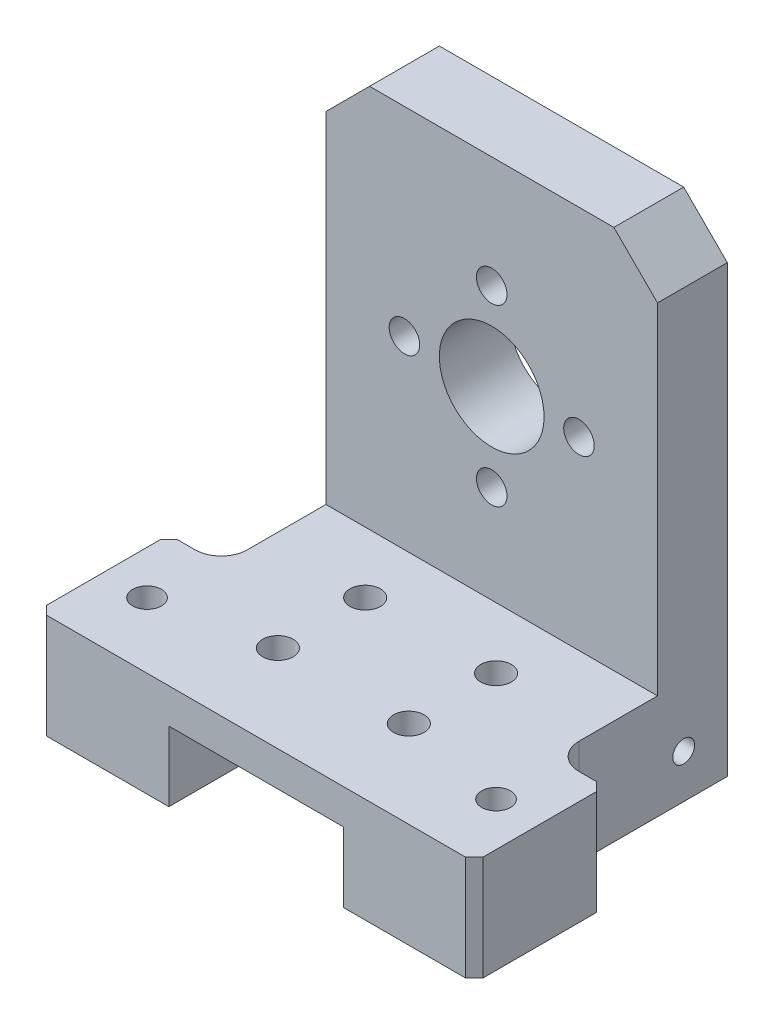
from build123d import *

# Parameters (mm, degrees)
SKETCH1_W             = 50
SKETCH1_H             = 56
SKETCH1_R             = 6
BOSS_EXTRUDE1_DEPTH   = 8
SKETCH2_W             = 50
SKETCH2_H             = 35
BOSS_EXTRUDE2_DEPTH   = 12
SKETCH3_W             = 20
SKETCH3_H             = 35
CUT_EXTRUDE1_DEPTH    = 8
SKETCH4_W             = 6
SKETCH4_H             = 44
CUT_EXTRUDE2_DEPTH    = 60
CHAMFER2_SIZE         = 5
SKETCH5_W             = 6
SKETCH5_H             = 20
CUT_EXTRUDE3_DEPTH    = 60
M4_TAPPED_HOLE1_D     = 3.3
FILLET1_R             = 3
SKETCH9_R             = 1.75
CUT_EXTRUDE4_DEPTH    = 10
SKETCH10_R            = 1.75
CUT_EXTRUDE5_DEPTH    = 10
M3_TAPPED_HOLE1_D     = 2.5
M3_TAPPED_HOLE1_DEPTH = 7.5
M3_TAPPED_HOLE1_TIP   = 0.751075774
CHAMFER3_SIZE         = 1


with BuildPart() as part:
    # Sketch1 → Boss-Extrude1 (new body)
    with BuildSketch(Plane.XY):
        Rectangle(SKETCH1_W, SKETCH1_H)
        with Locations((0, 5.2)):
            Circle(SKETCH1_R, mode=Mode.SUBTRACT)
    extrude(amount=BOSS_EXTRUDE1_DEPTH)

    # Sketch2 → Boss-Extrude2 (add)
    with BuildSketch(Plane.XZ.offset(28)):
        with Locations((0, 17.5)):
            Rectangle(SKETCH2_W, SKETCH2_H)
    extrude(amount=-BOSS_EXTRUDE2_DEPTH)

    # Sketch3 → Cut-Extrude1 (cut)
    with BuildSketch(Plane.XZ.offset(28)):
        with Locations((0, 17.5)):
            Rectangle(SKETCH3_W, SKETCH3_H)
    extrude(amount=-CUT_EXTRUDE1_DEPTH, mode=Mode.SUBTRACT)

    # Sketch4 → Cut-Extrude2 (cut)
    with BuildSketch(Plane.XY.offset(35)):
        with Locations((-22, 6)):
            Rectangle(SKETCH4_W, SKETCH4_H)
        with Locations((22, 6)):
            Rectangle(SKETCH4_W, SKETCH4_H)
    extrude(amount=-CUT_EXTRUDE2_DEPTH, mode=Mode.SUBTRACT)

    # Chamfer2
    chamfer2_edges = [part.edges().sort_by_distance(p)[0] for p in [
        (-19, 28, 4),
        (19, 28, 4),
    ]]
    chamfer(chamfer2_edges, length=CHAMFER2_SIZE)

    # Sketch5 → Cut-Extrude3 (cut)
    with BuildSketch(Plane(origin=(0, 28, 0), x_dir=(1, 0, 0), z_dir=(0, 1, 0))):
        with Locations((-22, -10)):
            Rectangle(SKETCH5_W, SKETCH5_H)
        with Locations((22, -10)):
            Rectangle(SKETCH5_W, SKETCH5_H)
    extrude(amount=-CUT_EXTRUDE3_DEPTH, mode=Mode.SUBTRACT)

    # M4 Tapped Hole1 (through all)
    with Locations(Plane(origin=(0, -28, 0), x_dir=(-1, 0, 0), z_dir=(0, -1, 0))):
        with Locations((20, -27.5), (-20, -27.5)):
            Hole(M4_TAPPED_HOLE1_D / 2)

    # Fillet1
    fillet1_edges = [part.edges().sort_by_distance(p)[0] for p in [
        (-19, -22, 20),
        (19, -22, 20),
    ]]
    fillet(fillet1_edges, radius=FILLET1_R)

    # Sketch9 → Cut-Extrude4 (cut)
    with BuildSketch(Plane(origin=(0, -16, 0), x_dir=(1, 0, 0), z_dir=(0, 1, 0))):
        with Locations(Location((-7.5, -15, 0), (0, 0, 270))):
            Circle(SKETCH9_R)
        with Locations(Location((7.5, -15, 0), (0, 0, 90))):
            Circle(SKETCH9_R)
        with Locations(Location((-7.5, -25, 0), (0, 0, 270))):
            Circle(SKETCH9_R)
        with Locations(Location((7.5, -25, 0), (0, 0, 90))):
            Circle(SKETCH9_R)
    extrude(amount=-CUT_EXTRUDE4_DEPTH, mode=Mode.SUBTRACT)

    # Sketch10 → Cut-Extrude5 (cut)
    with BuildSketch(Plane.XY.offset(8)):
        with Locations((10, 5.2)):
            Circle(SKETCH10_R)
        with Locations((0, 15.2)):
            Circle(SKETCH10_R)
        with Locations((-10, 5.2)):
            Circle(SKETCH10_R)
        with Locations((0, -4.8)):
            Circle(SKETCH10_R)
    extrude(amount=-CUT_EXTRUDE5_DEPTH, mode=Mode.SUBTRACT)

    # M3 Tapped Hole1
    with Locations(Plane(origin=(19, 0, 0), x_dir=(0, 0, -1), z_dir=(1, 0, 0))):
        with Locations((-5, -23)):
            Hole(M3_TAPPED_HOLE1_D / 2, depth=M3_TAPPED_HOLE1_DEPTH)
            with Locations((0, 0, -(M3_TAPPED_HOLE1_DEPTH + M3_TAPPED_HOLE1_TIP / 2))):  # 118° drill point
                Cone(0, M3_TAPPED_HOLE1_D / 2, M3_TAPPED_HOLE1_TIP, mode=Mode.SUBTRACT)

    # Chamfer3
    chamfer3_edges = [part.edges().sort_by_distance(p)[0] for p in [
        (-25, -22, 20),
        (25, -22, 20),
        (-25, -22, 35),
        (25, -22, 35),
    ]]
    chamfer(chamfer3_edges, length=CHAMFER3_SIZE)


solid = part.part
